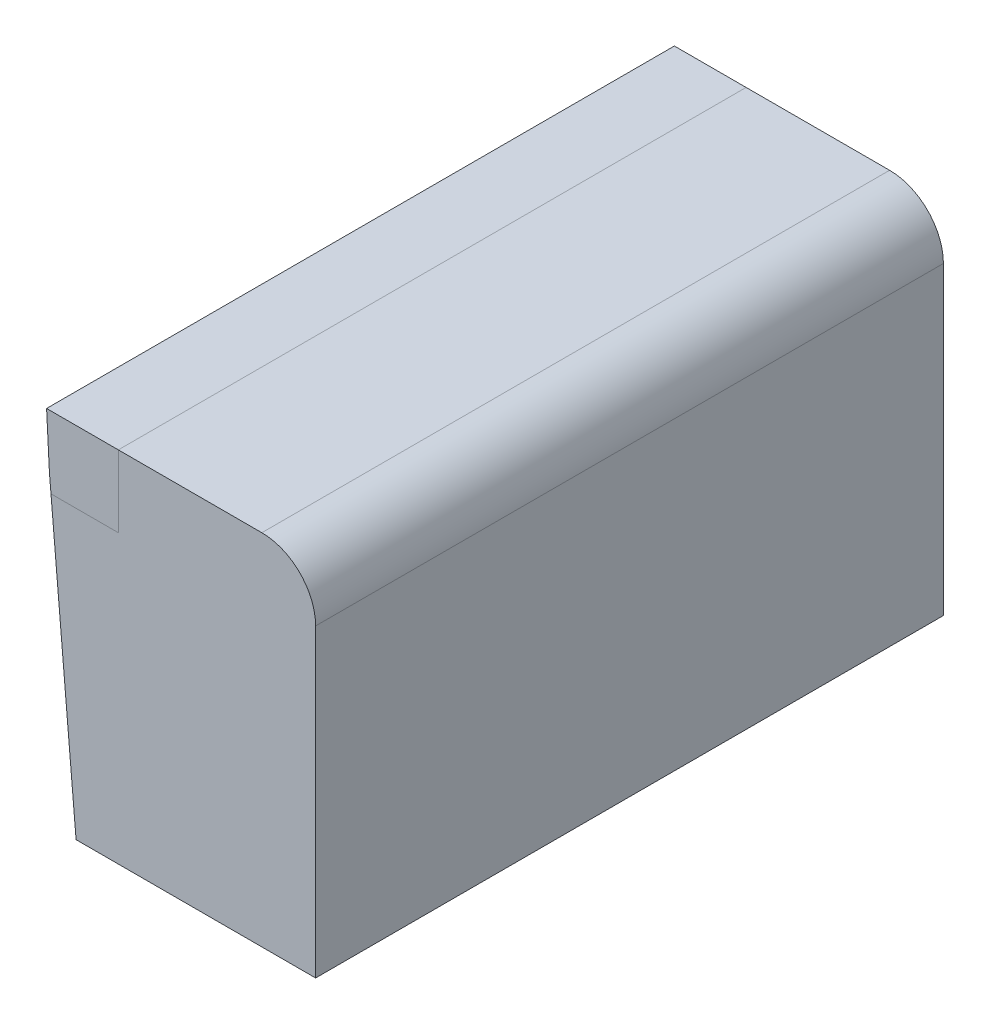
SolidWorks part; units mm, degrees
ref_plane "Front Plane" through (0, 0, 0) normal (0, 0, 1) x (1, 0, 0)
ref_plane "Top Plane" through (0, 0, 0) normal (0, 1, 0) x (1, 0, 0)
ref_plane "Right Plane" through (0, 0, 0) normal (1, 0, 0) x (0, 0, -1)
sketch "Sketch1" plane through (0, 0, 0) normal (0, 0, 1) x (1, 0, 0)
  line L0 (-14.8428, 17) -> (-15, 20)
  line L1 (0, 0) -> (-13.3555, 0)
  line L2 (0, 0) -> (0, 20)
  line L3 (0, 20) -> (-15, 20)
  line L4 (-13.3555, 0) -> (-14.8428, 17)
  dimension "D1" = 20
  dimension "D2" = 15
  dimension "D3" = 85
  dimension "D4" = 3
  dimension "D5" = 87
extrude "Boss-Extrude1" add sketch "Sketch1" along normal mid plane 35
sketch "Sketch2" plane through (0, 0, 17.5) normal (0, 0, 1) x (1, 0, 0)
  line L1 (-15, 20) -> (-11, 20)
  line L2 (-15, 20) -> (-15, 16)
  line L3 (-15, 16) -> (-11, 16)
  line L4 (-11, 20) -> (-11, 16)
  dimension "D1" = 4
  dimension "D2" = 4
split "Split1" trim tools "Sketch2" bodies to split 103 resulting bodies 104 105
hole_wizard "M6 Tapped Hole1" positions "Sketch4" profile "Sketch3" tap size "M6" standard "GB"
sketch "Sketch4" plane through (0, 0, 0) normal (0, -1, 0) x (1, 0, 0)
  line L0 (-6, 10) -> (-6, -10) construction
  line L3 (-6, 0) -> (0, 0) construction
  line L5 (0, 17.5) -> (0, -17.5) construction
  point P0 (-6, 10)
  point P1 (-6, -10)
  dimension "D1" = 20
  dimension "D2" = 6
sketch "Sketch3" plane through (-6, 0, 10) normal (1, 0, 0) x (0, 0, -1)
  line L0 (0, 0) -> (0, 16.5022)
  line L1 (0, 16.5022) -> (2.5, 15)
  line L2 (2.5, 15) -> (2.5, 0)
  line L5 (2.5, 0) -> (0, 0)
  line L10 (0, 16.5022) -> (-2.5, 15) construction
  line L11 (0, -6.35) -> (0, 107.95) construction
  dimension "螺纹孔钻头直径" = 5
  dimension "螺纹孔钻头深度" = 15
  dimension "导头角度" = 118
cosmetic thread "Hole cosmetic thread1" parameters "D1"=12, "D2"=6
cosmetic thread "Hole cosmetic thread2" parameters "D1"=12, "D2"=6
fillet "Fillet1" radius 3 1 edges at (0, 20, 0)
